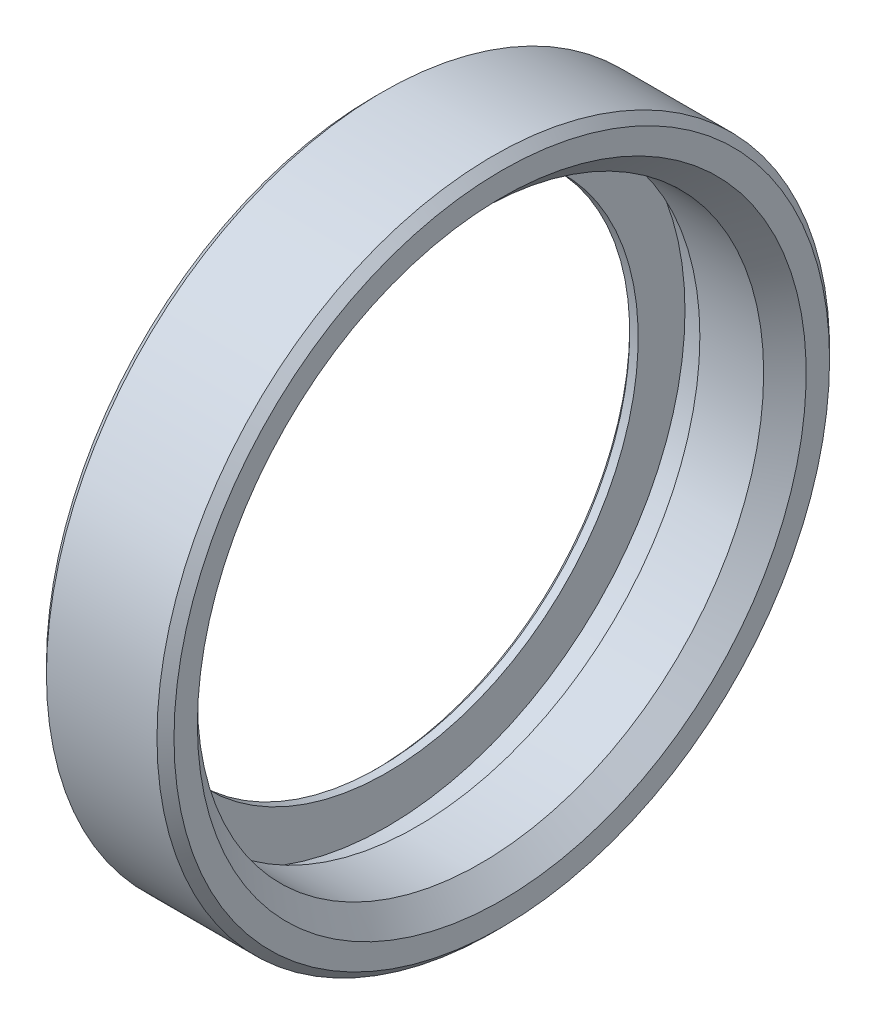
from build123d import *


with BuildPart() as part:
    # Sketch1 → Revolve1 (revolve)
    with BuildSketch(Plane.XY, mode=Mode.PRIVATE) as revolve1_sk:
        Polygon((1542.193616015, 1896.149332348), (1541.965999426, 1896.149332348), (1541.852191131, 1896.035524053), (1541.852191131, 1894.100783041), (1542.07980772, 1893.873166452), (1545.038823386, 1893.873166452), (1545.266439975, 1894.100783041), (1545.266439975, 1894.726728663), (1544.981919238, 1895.0112494), (1542.990274079, 1895.0112494), (1542.990274079, 1894.897441105), (1542.193616015, 1894.897441105), align=None)
        Polygon((1542.990274079, 1895.295770137), (1542.990274079, 1895.0112494), (1544.981919238, 1895.0112494), (1544.697398501, 1895.295770137), align=None)
    revolve(revolve1_sk.sketch.rotate(Axis((1539.352588353, 1902.873166452, 0), (1, 0, 0)), 270), axis=Axis((1539.352588353, 1902.873166452, 0), (1, 0, 0)))


solid = part.part
